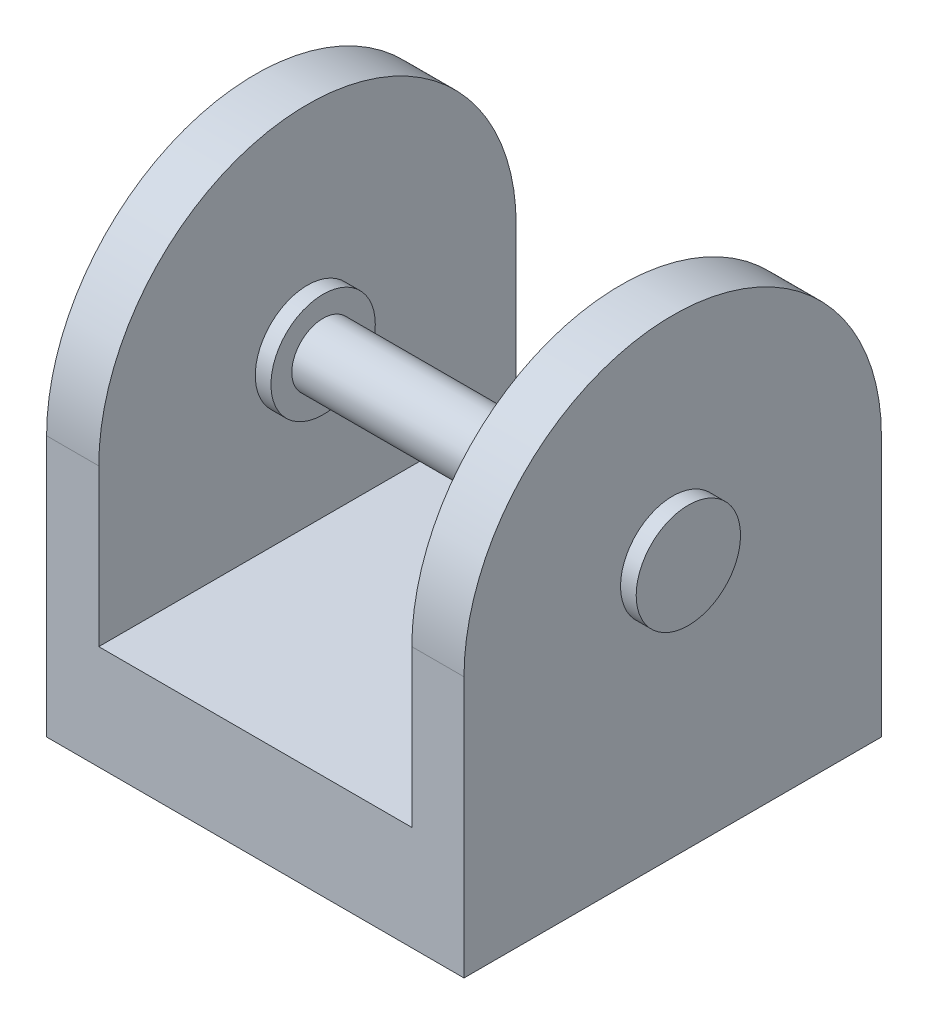
from build123d import *

# Parameters (mm, degrees)
SKETCH1_W           = 40
SKETCH1_H           = 40
BOSS_EXTRUDE1_DEPTH = 10
BOSS_EXTRUDE2_DEPTH = 5
SKETCH4_R           = 5
BOSS_EXTRUDE3_DEPTH = 4
BOSS_EXTRUDE4_REACH = 62.415
SKETCH5_R           = 3
SKETCH6_R           = 5
BOSS_EXTRUDE5_DEPTH = 5


with BuildPart() as part:
    # Sketch1 → Boss-Extrude1 (new body)
    with BuildSketch(Plane(origin=(0, 0, 0), x_dir=(1, 0, 0), z_dir=(0, 1, 0))):
        Rectangle(SKETCH1_W, SKETCH1_H)
    extrude(amount=BOSS_EXTRUDE1_DEPTH)

    # Sketch2 → Boss-Extrude2 (add)
    with BuildSketch(Plane(origin=(20, 0, 0), x_dir=(0, 0, -1), z_dir=(1, 0, 0))):
        with BuildLine():
            Line((-20, 10), (-20, 25))
            ThreePointArc((-20, 25), (0, 45), (20, 25))
            Line((20, 25), (20, 10))
            Line((20, 10), (-20, 10))
        make_face()
    boss_extrude2 = extrude(amount=-BOSS_EXTRUDE2_DEPTH)

    # Mirror1: Boss-Extrude2 across plane
    add(boss_extrude2.mirror(Plane(origin=(0, 0, 0), x_dir=(0, 0, 1), z_dir=(1, 0, 0))))

    # Sketch4 → Boss-Extrude3 (add, symmetric)
    with BuildSketch(Plane(origin=(17.5, 0, 0), x_dir=(0, 0, -1), z_dir=(1, 0, 0))):
        with Locations(Location((0, 25, 0), (0, 0, 180))):
            Circle(SKETCH4_R)
    boss_extrude3 = extrude(amount=BOSS_EXTRUDE3_DEPTH, both=True)

    # Mirror2: Boss-Extrude3 across plane
    add(boss_extrude3.mirror(Plane(origin=(0, 0, 0), x_dir=(0, 0, 1), z_dir=(1, 0, 0))))


with BuildPart() as body_2:

    # Sketch5 → Boss-Extrude4 (new, up to next)
    with BuildSketch(Plane.ZY.offset(-13.5), mode=Mode.PRIVATE) as boss_extrude4_sk1:
        with Locations((0, 25)):
            Circle(SKETCH5_R)
    boss_extrude4_tool1 = extrude(boss_extrude4_sk1.sketch, amount=BOSS_EXTRUDE4_REACH, mode=Mode.PRIVATE) - part.part
    add(boss_extrude4_tool1.solids().sort_by_distance((13.5, 25, 0))[0])


with BuildPart() as part_1:
    add(part.part)

    # Sketch6 → Boss-Extrude5 (add)
    with BuildSketch(Plane.ZY.offset(21.5)):
        with Locations((0, 25)):
            Circle(SKETCH6_R)
    extrude(amount=BOSS_EXTRUDE5_DEPTH)


solid = Compound([body_2.part, part_1.part])
